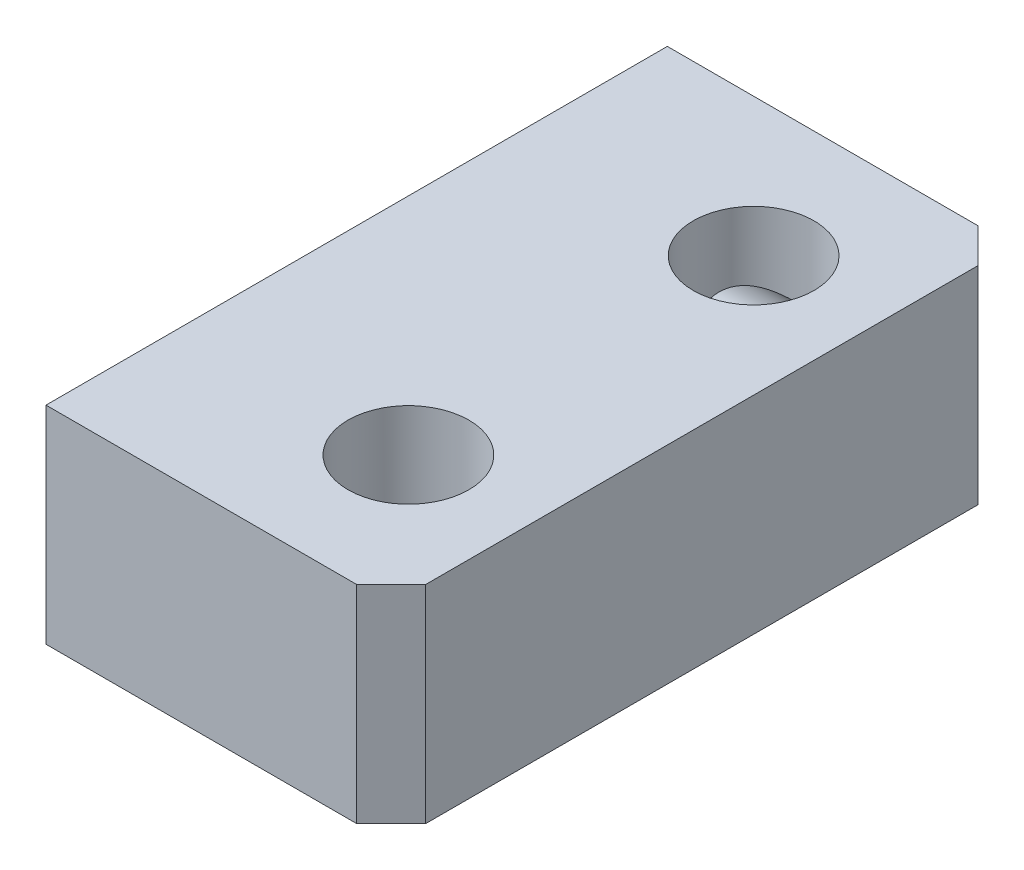
from build123d import *

# Parameters (mm, degrees)
SKETCH1_W               = 10
SKETCH1_H               = 18
BOSS_EXTRUDE1_DEPTH     = 6
SKETCH2_R               = 1.75
CUT_EXTRUDE1_DEPTH      = 10
CHAMFER1_SIZE           = 1
M2_5_TAPPED_HOLE1_D     = 2.05
M2_5_TAPPED_HOLE1_DEPTH = 6.35
M2_5_TAPPED_HOLE1_TIP   = 0.615882135


with BuildPart() as part:
    # Sketch1 → Boss-Extrude1 (new body)
    with BuildSketch(Plane(origin=(0, 0, 0), x_dir=(1, 0, 0), z_dir=(0, 1, 0))):
        Rectangle(SKETCH1_W, SKETCH1_H)
    extrude(amount=BOSS_EXTRUDE1_DEPTH)

    # Sketch2 → Cut-Extrude1 (cut)
    with BuildSketch(Plane(origin=(0, 6, 0), x_dir=(1, 0, 0), z_dir=(0, 1, 0))):
        with Locations(Location((1.5, 5, 0), (0, 0, 270))):
            Circle(SKETCH2_R)
        with Locations(Location((1.5, -5, 0), (0, 0, 270))):
            Circle(SKETCH2_R)
    extrude(amount=-CUT_EXTRUDE1_DEPTH, mode=Mode.SUBTRACT)

    # Chamfer1
    chamfer1_edges = [part.edges().sort_by_distance(p)[0] for p in [
        (5, 3, 9),
        (5, 3, -9),
    ]]
    chamfer(chamfer1_edges, length=CHAMFER1_SIZE)

    # M2.5 Tapped Hole1
    with Locations(Plane(origin=(-5, 3, -6), x_dir=(0, 0, -1), z_dir=(-1, 0, 0))):
        with Locations((0, 0), (-12, 0)):
            Hole(M2_5_TAPPED_HOLE1_D / 2, depth=M2_5_TAPPED_HOLE1_DEPTH)
            with Locations((0, 0, -(M2_5_TAPPED_HOLE1_DEPTH + M2_5_TAPPED_HOLE1_TIP / 2))):  # 118° drill point
                Cone(0, M2_5_TAPPED_HOLE1_D / 2, M2_5_TAPPED_HOLE1_TIP, mode=Mode.SUBTRACT)


solid = part.part
